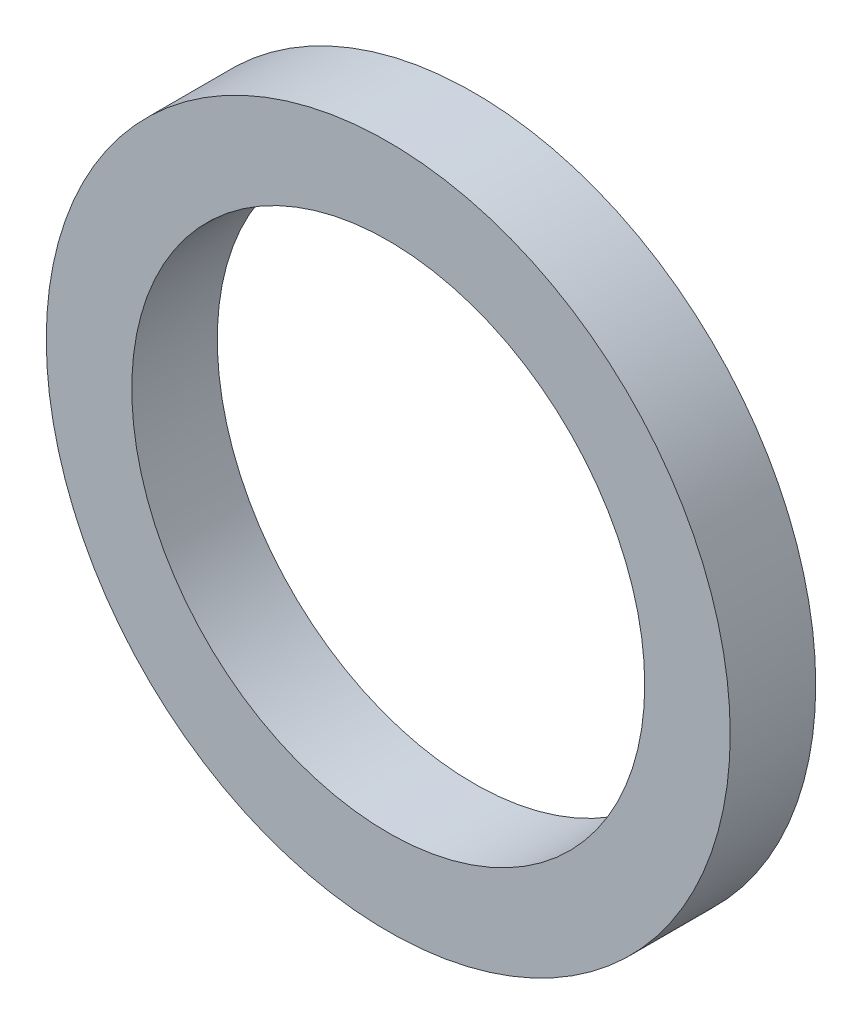
SolidWorks part; units mm, degrees
ref_plane "Front Plane" through (0, 0, 0) normal (0, 0, 1) x (1, 0, 0)
ref_plane "Top Plane" through (0, 0, 0) normal (0, 1, 0) x (1, 0, 0)
ref_plane "Right Plane" through (0, 0, 0) normal (1, 0, 0) x (0, 0, -1)
sketch "Sketch1" plane through (0, 0, 0) normal (0, 0, 1) x (1, 0, 0)
  circle A0 centre (0, 0) radius 6
  circle A1 centre (0, 0) radius 8
  dimension "D1" = 16
  dimension "D2" = 12
extrude "Boss-Extrude1" add sketch "Sketch1" along normal blind 2
